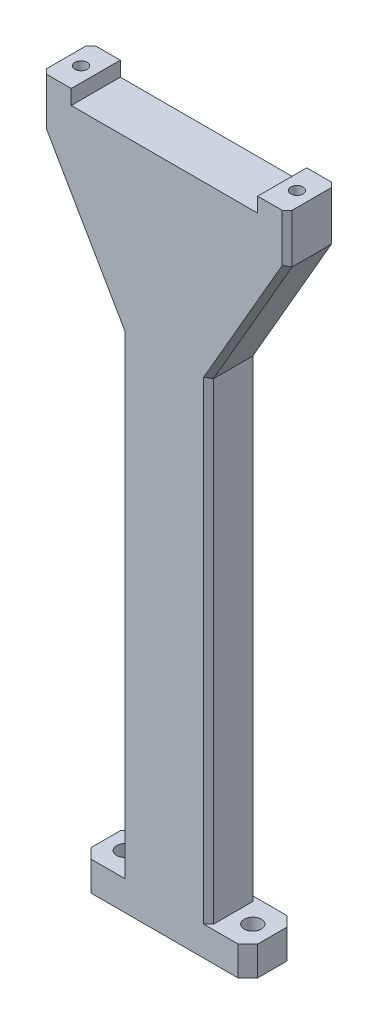
SolidWorks part; units mm, degrees
ref_plane "Front Plane" through (0, 0, 0) normal (0, 0, 1) x (1, 0, 0)
ref_plane "Top Plane" through (0, 0, 0) normal (0, 1, 0) x (1, 0, 0)
ref_plane "Right Plane" through (0, 0, 0) normal (1, 0, 0) x (0, 0, -1)
sketch "Sketch1" plane through (0, 0, 0) normal (0, 0, 1) x (1, 0, 0)
  line L1 (-25, 70) -> (25, 70)
  line L2 (-25, 70) -> (-25, -70)
  line L3 (-25, -70) -> (25, -70)
  line L4 (25, 70) -> (25, -70)
  line L5 (-25, 70) -> (25, -70) construction
  line L6 (-25, -70) -> (25, 70) construction
  point P0 (0, 0)
  dimension "D1" = 140
  dimension "D2" = 50
extrude "Boss-Extrude1" add sketch "Sketch1" along normal mid plane 10
sketch "Sketch2" plane through (0, 0, 5) normal (0, 0, 1) x (1, 0, 0)
  line L0 (-25, 60) -> (-9, 32.2872)
  line L1 (-25, 70) -> (-25, -70) construction
  line L2 (-9, 32.2872) -> (-9, -64)
  line L3 (-9, -64) -> (-17, -64)
  line L4 (-17, -64) -> (-17, -70)
  line L5 (-25, -70) -> (25, -70) construction
  line L6 (-17, -70) -> (-25, -70)
  line L7 (-25, -70) -> (-25, 60)
  line L8 (25, 70) -> (-25, 70) construction
  line L9 (0, 0) -> (0, 60) construction
  dimension "D1" = 10
  dimension "D2" = 30
  dimension "D3" = 6
  dimension "D4" = 8
  dimension "D5" = 16
extrude "Cut-Extrude1" cut sketch "Sketch2" against normal through all
mirror "Mirror1" about plane through (0, 0, 0) normal (1, 0, 0) of "Cut-Extrude1"
sketch "Sketch3" plane through (0, 0, 5) normal (0, 0, 1) x (1, 0, 0)
  line L0 (25, 70) -> (-25, 70) construction
  line L1 (-19, 70) -> (19, 70)
  line L2 (-19, 70) -> (-19, 67)
  line L3 (-19, 67) -> (19, 67)
  line L4 (19, 70) -> (19, 67)
  line L5 (-19, 70) -> (19, 67) construction
  line L6 (-19, 67) -> (19, 70) construction
  point P0 (0, 68.5)
  dimension "D1" = 38
  dimension "D2" = 3
extrude "Cut-Extrude2" cut sketch "Sketch3" against normal through all
hole_wizard "M3 Tapped Hole1" positions "Sketch5" profile "Sketch4" tap size "M3" standard "Gb"
sketch "Sketch5" plane through (0, 70, 0) normal (0, 1, 0) x (1, 0, 0)
  line L0 (0, 0) -> (0, 8.6428) construction
  line L2 (-25, -5) -> (-25, 5) construction
  point P0 (-22, 0)
  point P2 (22, 0)
  dimension "D1" = 3
sketch "Sketch4" plane through (-22, 70, 0) normal (1, 0, 0) x (0, 0, 1)
  line L0 (0, 0) -> (0, 9.2511)
  line L1 (0, 9.2511) -> (1.25, 8.5)
  line L2 (1.25, 8.5) -> (1.25, 0)
  line L5 (1.25, 0) -> (0, 0)
  line L10 (0, 9.2511) -> (-1.25, 8.5) construction
  line L11 (0, -6.35) -> (0, 107.95) construction
  dimension "螺纹孔钻头直径" = 2.5
  dimension "螺纹孔钻头深度" = 8.5
  dimension "导头角度" = 118
cosmetic thread "Hole Thread1" parameters "D1"=6, "D2"=3
cosmetic thread "Hole Thread2" parameters "D1"=6, "D2"=3
hole_wizard "Ø3.5 (3.5) Diameter Hole1" positions "Sketch7" profile "Sketch6" hole size "Ø3.5" standard "Gb"
sketch "Sketch7" plane through (0, -70, 0) normal (0, -1, 0) x (-1, 0, 0)
  line L0 (0, 0) -> (0, -7.6569) construction
  line L2 (17, 5) -> (17, -5) construction
  point P0 (13, 0)
  point P2 (-13, 0)
  dimension "D1" = 4
sketch "Sketch6" plane through (-13, -70, 0) normal (1, 0, 0) x (0, 0, -1)
  line L0 (0, 0) -> (0, 6)
  line L1 (0, 6) -> (1.75, 6)
  line L2 (1.75, 6) -> (1.75, 0)
  line L5 (1.75, 0) -> (0, 0)
  line L11 (0, -6.35) -> (0, 107.95) construction
  dimension "通孔孔直径" = 3.5
  dimension "通孔孔深度" = 6
chamfer "Chamfer1" distance 2 angle 45 4 edges at (-17, -67, -5) (-17, -67, 5) (17, -67, -5) (17, -67, 5)
chamfer "Chamfer2" distance 1 angle 45 12 edges at (-25, 65, -5) (-17, 46.1436, -5) (-9, -15.8564, -5) (-25, 65, 5) (-17, 46.1436, 5) (-9, -15.8564, 5) (25, 65, -5) (17, 46.1436, -5) (9, -15.8564, -5) (25, 65, 5) (17, 46.1436, 5) (9, -15.8564, 5)
